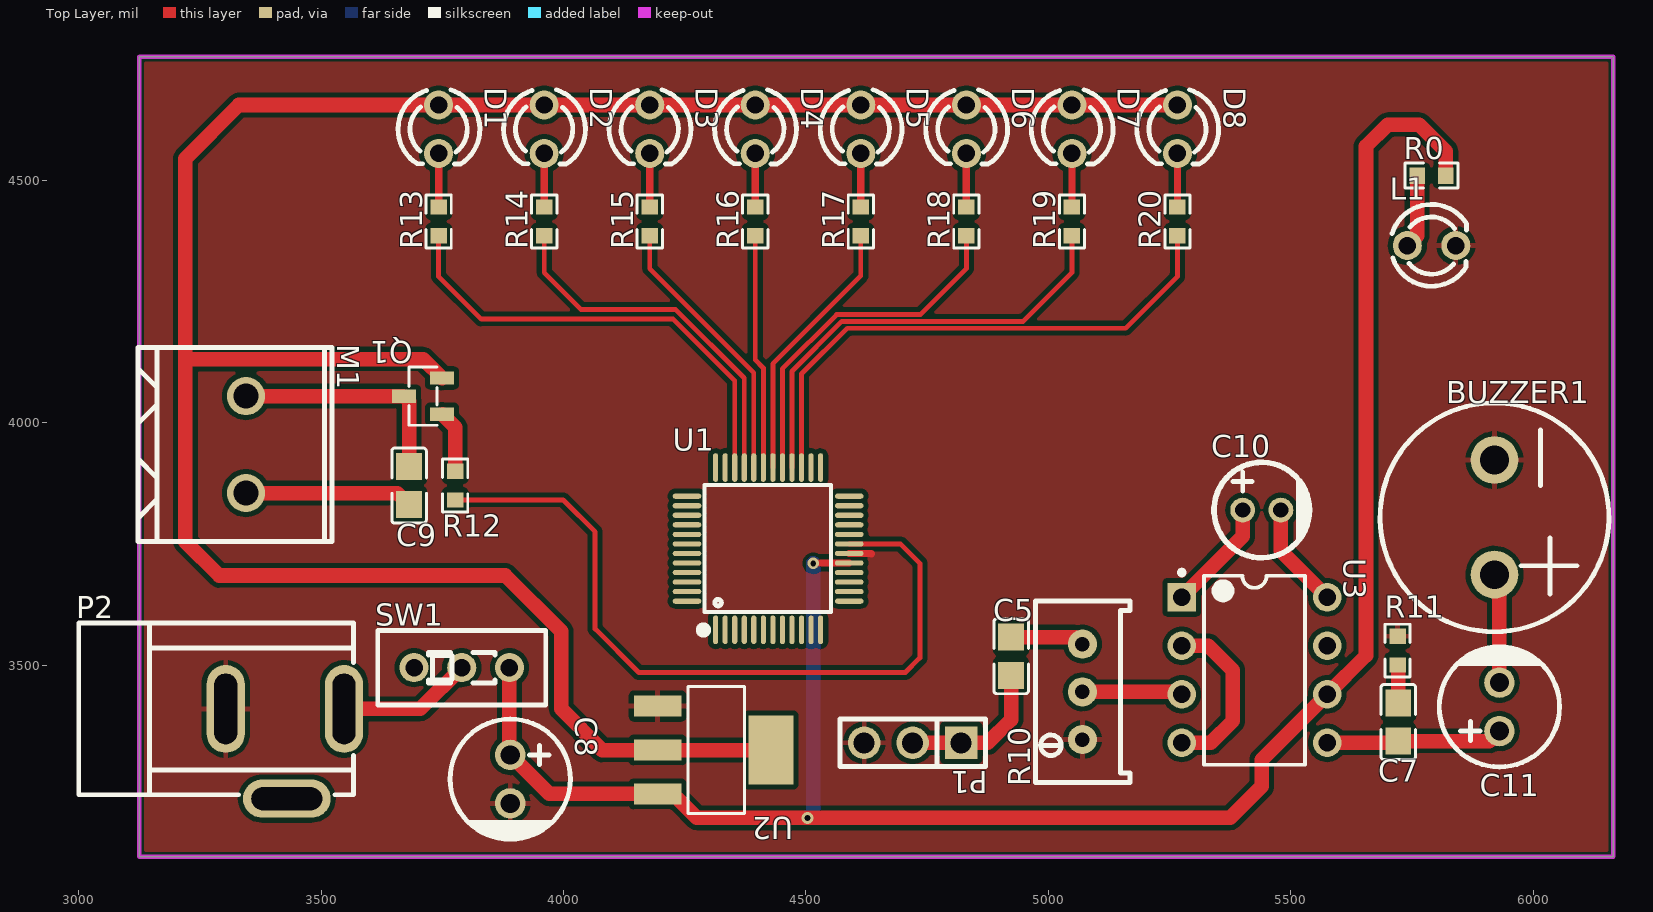
[diagram p0: Top Layer view]
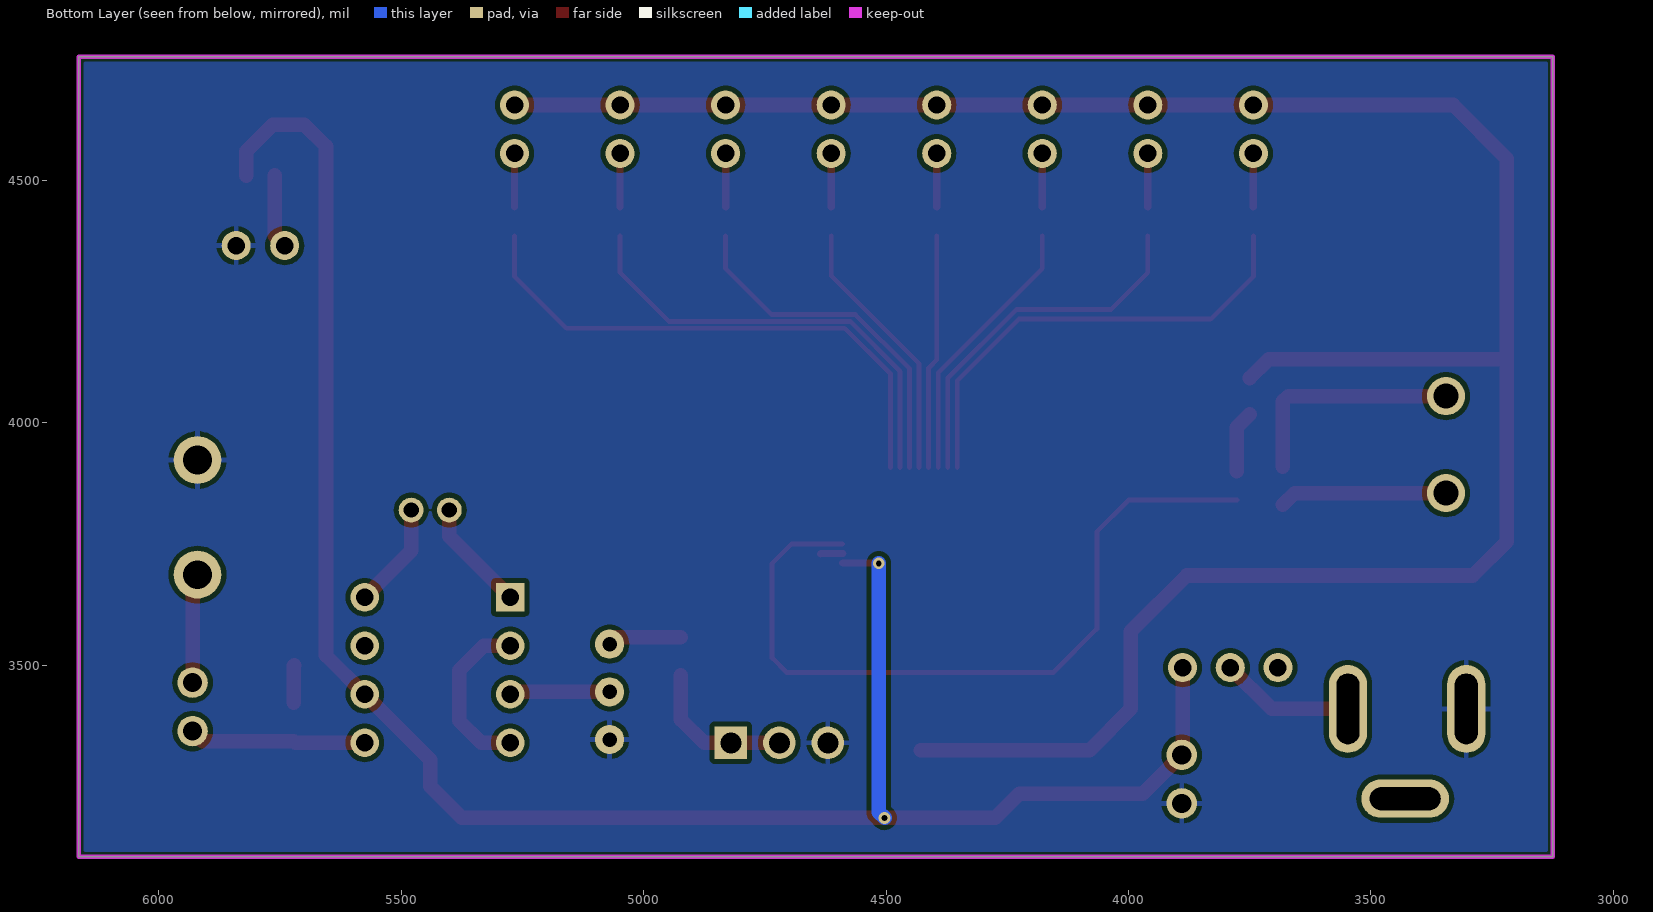
[diagram p1: Bottom Layer view, seen from below]
# Altium PCB MISC52120.pcbdoc
Units mil, origin at the board's own origin, x right, y up, seen from the top; angles counter-clockwise.
Board outline 3040 x 1650 mil, 2 copper layers (Top Layer, Bottom Layer), stack 62.206 mil thick; 36 components, 35 nets, 131 pads, 2 vias.

## Layer stack, top to bottom
Top Solder Mask Layer: solder mask 0.394, Dk 3.3
Top Layer: signal copper 1.379
Dielectric1: surface 59.449, FR4, Dk 4.5
Bottom Layer: signal copper 1.378
Bottom Solder Mask Layer: solder mask 0.394, Dk 3.3

## Board outline
3125,4755 3125,3105 6165,3105 6165,4755

## Design rules (kind name [scope] priority, off if disabled: settings)
BoardOutlineClearance copperThickness2oz_1 [All] p2 off: genericclearance=7.99 ignorepadtopadclearanceinfootprint=FALSE except(0: Arc-SplitContinuation Track-SplitContinuation SMDPad-SplitContinuation THPad-SplitContinuation Via-SplitContinuation Fill-SplitContinuation Region-SplitContinuation Poly-SplitContinuation Text-SplitContinuation Hole-SplitContinuation; 5.98: Arc-CutoutEdge Track-CutoutEdge SMDPad-CutoutEdge THPad-CutoutEdge Via-CutoutEdge Text-CutoutEdge; 6.9: Hole-OutlineEdge Hole-CutoutEdge; 10: Poly-OutlineEdge Poly-CutoutEdge; 11.81: Arc-OutlineEdge Track-OutlineEdge SMDPad-OutlineEdge THPad-OutlineEdge Via-OutlineEdge Fill-OutlineEdge Region-OutlineEdge Text-OutlineEdge Fill-CutoutEdge Region-CutoutEdge)
BoardOutlineClearance Plane_innerPlane_1 [All] p4 off: genericclearance=4.02 ignorepadtopadclearanceinfootprint=FALSE except(0: Arc-SplitContinuation Track-SplitContinuation SMDPad-SplitContinuation THPad-SplitContinuation Via-SplitContinuation Fill-SplitContinuation Region-SplitContinuation Poly-SplitContinuation Text-SplitContinuation Hole-SplitContinuation; 5.98: Arc-CutoutEdge Track-CutoutEdge SMDPad-CutoutEdge THPad-CutoutEdge Via-CutoutEdge Text-CutoutEdge; 6.9: Hole-OutlineEdge Hole-CutoutEdge; 10: Poly-OutlineEdge Poly-CutoutEdge; 11.81: Arc-OutlineEdge Track-OutlineEdge SMDPad-OutlineEdge THPad-OutlineEdge Via-OutlineEdge Fill-OutlineEdge Region-OutlineEdge Text-OutlineEdge Fill-CutoutEdge Region-CutoutEdge)
BoardOutlineClearance Copper_copperRegion_1 [All] p6 off: genericclearance=4.02 ignorepadtopadclearanceinfootprint=FALSE except(0: Arc-SplitContinuation Track-SplitContinuation SMDPad-SplitContinuation THPad-SplitContinuation Via-SplitContinuation Fill-SplitContinuation Region-SplitContinuation Poly-SplitContinuation Text-SplitContinuation Hole-SplitContinuation; 5.98: Arc-CutoutEdge Track-CutoutEdge SMDPad-CutoutEdge THPad-CutoutEdge Via-CutoutEdge Text-CutoutEdge; 6.9: Hole-OutlineEdge Hole-CutoutEdge; 10: Poly-OutlineEdge Poly-CutoutEdge; 11.81: Arc-OutlineEdge Track-OutlineEdge SMDPad-OutlineEdge THPad-OutlineEdge Via-OutlineEdge Fill-OutlineEdge Region-OutlineEdge Text-OutlineEdge Fill-CutoutEdge Region-CutoutEdge)
BoardOutlineClearance copperThickness1oz_1 [All] p8: genericclearance=4.02 ignorepadtopadclearanceinfootprint=FALSE except(0: Arc-SplitContinuation Track-SplitContinuation SMDPad-SplitContinuation THPad-SplitContinuation Via-SplitContinuation Fill-SplitContinuation Region-SplitContinuation Poly-SplitContinuation Text-SplitContinuation Hole-SplitContinuation; 5.98: Arc-CutoutEdge Track-CutoutEdge SMDPad-CutoutEdge THPad-CutoutEdge Via-CutoutEdge Text-CutoutEdge; 6.9: Hole-OutlineEdge Hole-CutoutEdge; 10: Poly-OutlineEdge Poly-CutoutEdge; 11.81: Arc-OutlineEdge Track-OutlineEdge SMDPad-OutlineEdge THPad-OutlineEdge Via-OutlineEdge Fill-OutlineEdge Region-OutlineEdge Text-OutlineEdge Fill-CutoutEdge Region-CutoutEdge)
Clearance copperThickness2oz [All] p1 off: gap=7.99 ignorepadtopadclearanceinfootprint=FALSE except(5.98: SMDPad-Track SMDPad-SMDPad THPad-Track SMDPad-THPad THPad-THPad Track-Via SMDPad-Via THPad-Via Via-Via Fill-SMDPad Region-SMDPad Fill-THPad Region-THPad Fill-Via Region-Via Fill-Fill Fill-Region Region-Region Arc-Track Arc-SMDPad Arc-THPad Arc-Via Fill-Arc Region-Arc Arc-Arc Text-Track SMDPad-Text Text-THPad Text-Via Fill-Text Region-Text Arc-Text Text-Text; 6.9: Hole-Track Hole-SMDPad Hole-THPad Hole-Via Fill-Hole Region-Hole Hole-Arc Hole-Text; 10: Poly-Track Poly-SMDPad Poly-THPad Poly-Via Poly-Fill Poly-Region Poly-Poly Poly-Arc Poly-Text Poly-Hole; 11.81: Fill-Track Region-Track)
Clearance Plane_innerPlane [All] p3 off: gap=4.02 ignorepadtopadclearanceinfootprint=FALSE except(5.98: SMDPad-Track SMDPad-SMDPad THPad-Track SMDPad-THPad THPad-THPad Track-Via SMDPad-Via THPad-Via Via-Via Fill-SMDPad Region-SMDPad Fill-THPad Region-THPad Fill-Via Region-Via Fill-Fill Fill-Region Region-Region Arc-Track Arc-SMDPad Arc-THPad Arc-Via Fill-Arc Region-Arc Arc-Arc Text-Track SMDPad-Text Text-THPad Text-Via Fill-Text Region-Text Arc-Text Text-Text; 6.9: Hole-Track Hole-SMDPad Hole-THPad Hole-Via Fill-Hole Region-Hole Hole-Arc Hole-Text; 10: Poly-Track Poly-SMDPad Poly-THPad Poly-Via Poly-Fill Poly-Region Poly-Poly Poly-Arc Poly-Text Poly-Hole; 11.81: Fill-Track Region-Track)
Clearance Copper_copperRegion [All] p5 off: gap=4.02 ignorepadtopadclearanceinfootprint=FALSE except(5.98: SMDPad-Track SMDPad-SMDPad THPad-Track SMDPad-THPad THPad-THPad Track-Via SMDPad-Via THPad-Via Via-Via Fill-SMDPad Region-SMDPad Fill-THPad Region-THPad Fill-Via Region-Via Fill-Fill Fill-Region Region-Region Arc-Track Arc-SMDPad Arc-THPad Arc-Via Fill-Arc Region-Arc Arc-Arc Text-Track SMDPad-Text Text-THPad Text-Via Fill-Text Region-Text Arc-Text Text-Text; 6.9: Hole-Track Hole-SMDPad Hole-THPad Hole-Via Fill-Hole Region-Hole Hole-Arc Hole-Text; 10: Poly-Track Poly-SMDPad Poly-THPad Poly-Via Poly-Fill Poly-Region Poly-Poly Poly-Arc Poly-Text Poly-Hole; 11.81: Fill-Track Region-Track)
Clearance copperThickness1oz [All] p7: gap=4.02 ignorepadtopadclearanceinfootprint=FALSE except(5.98: SMDPad-Track SMDPad-SMDPad THPad-Track SMDPad-THPad THPad-THPad Track-Via SMDPad-Via THPad-Via Via-Via Fill-SMDPad Region-SMDPad Fill-THPad Region-THPad Fill-Via Region-Via Fill-Fill Fill-Region Region-Region Arc-Track Arc-SMDPad Arc-THPad Arc-Via Fill-Arc Region-Arc Arc-Arc Text-Track SMDPad-Text Text-THPad Text-Via Fill-Text Region-Text Arc-Text Text-Text; 6.9: Hole-Track Hole-SMDPad Hole-THPad Hole-Via Fill-Hole Region-Hole Hole-Arc Hole-Text; 10: Poly-Track Poly-SMDPad Poly-THPad Poly-Via Poly-Fill Poly-Region Poly-Poly Poly-Arc Poly-Text Poly-Hole; 11.81: Fill-Track Region-Track)
DiffPairsRouting differentialPair [All] p1: maxlimit=6 minlimit=6 mostfreqgap=6 toplayer_minwidth=5 toplayer_prefwidth=10 toplayer_maxwidth=100 toplayer_mingap=6 toplayer_prefgap=6 toplayer_maxgap=6 bottomlayer_minwidth=5 bottomlayer_prefwidth=10 bottomlayer_maxwidth=100 bottomlayer_mingap=6 bottomlayer_prefgap=6 bottomlayer_maxgap=6 maxuncoupledlength=10
HoleToHoleClearance otherClearance [All] p1: gap=11.81 allowstackedmicrovias=TRUE
Length netLength [All] p1: minlimit=0 maxlimit=0
PasteMaskExpansion pasteMaskExpansion [All] p1: expansion=0
PlaneConnect innerPlane [All] p1: planeconnectstyle=Relief reliefexpansion=20 reliefentries=4 reliefconductorwidth=10 reliefairgap=10
PolygonConnect copperRegion [All] p1: connectstyle=Relief reliefconductorwidth=10 reliefentries=4 polygonreliefangle="90 Angle" airgapwidth=10 via.connectstyle=Relief via.reliefconductorwidth=10 via.reliefentries=4 via.polygonreliefangle="90 Angle" via.airgapwidth=10
RoutingVias viaSize [All] p1: holewidth=12.01 width=24.02 viastyle="Through Hole" minholewidth=11.81 minwidth=19.68 maxholewidth=248.03 maxwidth=393.7
SolderMaskExpansion solderMaskExpansion [IsVia] p1: expansion=-1000 istentingtop=TRUE
SolderMaskExpansion solderMaskExpansion [All] p2: expansion=2 istentingtop=FALSE
Width copperThickness2oz_2 [All] p1 off: maxlimit=100 minlimit=8 preferedwidth=10
Width copperThickness1oz_2 [All] p2: maxlimit=100 minlimit=5 preferedwidth=10

## Components (designator, comment, footprint, x,y, rotation, side; value= is the part's Value field where it differs from the comment)
BUZZER1 "buzzer" BUZ-TH_BD12.0-P6.00-D0.9-RD 5920,3805 r270 top
C5 "104" C0805 4923.07,3518.52 r270 top
C7 "104" C0805 5721.62,3382.82 r90 top
C8 "220uF" CAP-TH_BD6.3-P2.50-D1.0-FD 3890,3265 r270 top
C9 "104" C0805 3681.31,3870.47 r90 top
C10 "10uF" CAP-TH_BD5.0-P2.00-D0.8-FD 5440,3820 r0 top
C11 "220uF" CAP-TH_BD6.3-P2.50-D1.0-FD 5930.17,3414.15 r90 top
D1 "LED0" LED_TH-3mm 3742.34,4605.45 r270 top
D2 "LED0" LED_TH-3mm 3960.03,4605.45 r270 top
D3 "LED0" LED_TH-3mm 4177.71,4605.45 r270 top
D4 "LED0" LED_TH-3mm 4395.39,4605.45 r270 top
D5 "LED0" LED_TH-3mm 4613.07,4605.45 r270 top
D6 "LED0" LED_TH-3mm 4830.75,4605.45 r270 top
D7 "LED0" LED_TH-3mm 5048.44,4605.45 r270 top
D8 "LED0" LED_TH-3mm 5266.12,4605.45 r270 top
L1 "RED" LED_TH-3mm 5790.19,4365.45 r0 top
M1 "Motor" CONN-TH_2P-P5.08-WJ500V-5.08-2P 3345,3955 r270 top
P1 "" HDR-TH_3P-P2.54-V-M 4720,3340 r180 top
P2 "DC005" DC-IN-TH_DC005 3425.19,3317.31 r0 top
Q1 "9012" SOT-23-3_L2.9-W1.3-P1.90-LS2.4-BR 3710,4055 r0 top
R0 "1K" R0603 5790,4510 r0 top
R10 "10kΩ" R_3296 5065,3445 r90 top
R11 "4.7" R0603 5720,3530 r270 top
R12 "1K" R0603 3776.31,3870.47 r270 top
R13 "1K" R0603 3742.34,4415.34 r90 top
R14 "1K" R0603 3960.03,4415.34 r90 top
R15 "1K" R0603 4177.71,4415.34 r90 top
R16 "1K" R0603 4395.39,4415.34 r90 top
R17 "1K" R0603 4613.07,4415.34 r90 top
R18 "1K" R0603 4830.75,4415.34 r90 top
R19 "1K" R0603 5048.44,4415.34 r90 top
R20 "1K" R0603 5266.12,4415.34 r90 top
SW1 "Switch" SW-TH_SS-12D01-GX 3790,3495 r0 top
U1 "STM32F103" LQFP-48_L7.0-W7.0-P0.50-LS9.0-BL 4421.86,3740.34 r0 top
U2 "AMS1117" SOT-223-3_L6.5-W3.4-P2.30-LS7.0-BR 4310.89,3325 r180 top
U3 "LM386N-3/NOPB" DIP-8_L9.8-W6.6-P2.54-LS7.6-BL 5425,3490 r270 top

## Footprints (in the part's own frame and the unit in brackets; to place one, negate y for a bottom-side part, rotate by r counter-clockwise, add the part's x,y. Pads: shape width x height; smd on the part's side, far side on the other; paste and mask are expansions set on the pad)
BUZ-TH_BD12.0-P6.00-D0.9-RD [mm]
  round 2.5 hole 1.5 paste+0 mask+0.05: 1(-3,0) 2(3,0)
  silkscreen extent -5.99,-5.99 5.99,5.99
C0805 [mm]
  rect 1.41x1.35 smd paste-100 mask+0.051: 1(-1,0) 2(1,0)
  silkscreen extent -1.96,-0.9 1.96,0.9
CAP-TH_BD5.0-P2.00-D0.8-FD [mm]
  round 1.3 hole 0.8: 1(-1,0) 2(1,0)
  silkscreen extent -2.5,-2.5 2.5,2.5
CAP-TH_BD6.3-P2.50-D1.0-FD [mm]
  round 1.6 hole 1: 1(-1.27,0) 2(1.27,0)
  silkscreen extent -3.15,-3.15 3.17,3.15
CONN-TH_2P-P5.08-WJ500V-5.08-2P [mm]
  round 2 hole 1.3 copper offset 0,0 paste+0 mask+0.051: 1(-2.54,0) 2(2.54,0)
  silkscreen extent -5.08,-5.66 5.08,4.5
DC-IN-TH_DC005 [mm]
  oval 2x4.6 hole 1.2 slot 3.7 at 90 deg: 1(3.1,2.35) 2(-3.1,2.35)
  oval 4.6x2 hole 1.2 slot 3.7 at 0 deg: 3(0.1,-2.35)
  silkscreen extent -10.8,-2.15 3.6,6.85
DIP-8_L9.8-W6.6-P2.54-LS7.6-BL [mm]
  rect 1.5x1.5 hole 0.9: 1(-3.81,-3.81)
  round 1.5 hole 0.9: 2(-1.27,-3.81) 3(1.27,-3.81) 4(3.81,-3.81) 5(3.81,3.81) 6(1.27,3.81) 7(-1.27,3.81) 8(-3.81,3.81)
  silkscreen extent -5.23,-3.93 4.96,2.65
HDR-TH_3P-P2.54-V-M [mm]
  rect 1.7x1.7 hole 1.1: 1(-2.54,0)
  round 1.7 hole 1.1: 2(0,0) 3(2.54,0)
  silkscreen extent -3.81,-1.25 3.81,1.25
LED_TH-3mm [mil]
  round 60 hole 36 paste+0 mask+2: 1(-50,0) 2(50,0)
  silkscreen extent -81,-84 72,85
LQFP-48_L7.0-W7.0-P0.50-LS9.0-BL [mm]
  oval 0.27x1.5 smd paste+0 mask+0.05: 1(-2.75,-4.25) 2(-2.25,-4.25) 3(-1.75,-4.25) 4(-1.25,-4.25) 5(-0.75,-4.25) 6(-0.25,-4.25) 7(0.25,-4.25) 8(0.75,-4.25) 9(1.25,-4.25) 10(1.75,-4.25) 11(2.25,-4.25) 12(2.75,-4.25) 25(2.75,4.25) 26(2.25,4.25) 27(1.75,4.25) 28(1.25,4.25) 29(0.75,4.25) 30(0.25,4.25) 31(-0.25,4.25) 32(-0.75,4.25) 33(-1.25,4.25) 34(-1.75,4.25) 35(-2.25,4.25) 36(-2.75,4.25)
  oval 1.5x0.27 smd paste+0 mask+0.05: 13(4.25,-2.75) 14(4.25,-2.25) 15(4.25,-1.75) 16(4.25,-1.25) 17(4.25,-0.75) 18(4.25,-0.25) 19(4.25,0.25) 20(4.25,0.75) 21(4.25,1.25) 22(4.25,1.75) 23(4.25,2.25) 24(4.25,2.75) 37(-4.25,2.75) 38(-4.25,2.25) 39(-4.25,1.75) 40(-4.25,1.25) 41(-4.25,0.75) 42(-4.25,0.25) 43(-4.25,-0.25) 44(-4.25,-0.75) 45(-4.25,-1.25) 46(-4.25,-1.75) 47(-4.25,-2.25) 48(-4.25,-2.75)
  silkscreen extent -3.59,-4.46 3.3,3.34
R0603 [mil]
  rect 31.75x34.02 smd paste-3937.01 mask+2: 1(-29.66,0) 2(29.66,0)
  silkscreen extent -55,-26 55,26
R_3296 [mil]
  round 60 hole 30 paste+0 mask+2: 1(-98.4,-5) 2(0,-5) 3(98.4,-5)
  silkscreen extent -187,-103 187,92
SOT-23-3_L2.9-W1.3-P1.90-LS2.4-BR [mm]
  rect 1.25x0.7 smd: 1(1,-0.95) 2(1,0.95) 3(-1,0)
  silkscreen extent -0.73,-1.53 0.73,1.53
SOT-223-3_L6.5-W3.4-P2.30-LS7.0-BR [mm]
  rect 2.5x1.1 smd: 1(2.97,-2.3) 2(2.97,0) 3(2.97,2.3)
  rect 2.34x3.6 smd: 4(-2.97,0)
  silkscreen extent -1.57,-3.33 1.37,3.33
SW-TH_SS-12D01-GX [mil]
  round 60 hole 36: 1(-98.43,0) 2(-0.01,0) 3(98.42,0)
  silkscreen extent -173,-77 173,77

## Via types
v1: diameter 24, hole 12, Top Layer to Bottom Layer, 2 vias

## Nets (pads, with @x,y where several pads share a name; then routed paths per layer and width w, separated by ;. In a path a pad name is that pad's centre, name@x,y a point inside that pad or via, vN(x,y) a via of type N, cw(c..) or ccw(c..) an arc to the next point about the centre after c; other vN are vias at no path point)
3V: D1.1 D2.1 D3.1 D4.1 D5.1 D6.1 D7.1 D8.1 Q1.2 U2.2 U2.4 | length 4907
  Top Layer w30: Q1.2 3710.56,4131.21 3220,4131.21 ; U2.4 U2.2 4080,3325 3995,3410 3995,3570 3880,3685 3290,3685 3220,3755 3220,4131.21 ; D8.1 D7.1 D6.1 D5.1 D4.1 D3.1 D2.1 D1.1 3330.45,4655.45 3220,4545 3220,4131.21
$1N159: L1.1 R0.1 | length 152.9
  Top Layer w30: L1.1 5760.34,4385.6 R0.1
$1N348: Q1.1 R12.1 | length 128.6
  Top Layer w30: Q1.1 3776.31,3990.66 R12.1
$1N425: C9.2 M1.1 Q1.3 | length 475.2
  Top Layer w30: M1.1 Q1.3 ; Q1.3 3681.31,4044.32 C9.2
$1N506: C9.1 M1.2 | length 346.2
  Top Layer w30: M1.2 3657.42,3854.99 C9.1
$1N2273: D1.2 R13.2 | length 110.4
  Top Layer w15: R13.2 D1.2
$1N2330: D2.2 R14.2 | length 110.4
  Top Layer w15: R14.2 D2.2
$1N2379: D3.2 R15.2 | length 110.4
  Top Layer w15: R15.2 D3.2
$1N2428: D4.2 R16.2 | length 110.4
  Top Layer w15: R16.2 D4.2
$1N2477: D5.2 R17.2 | length 110.4
  Top Layer w15: R17.2 D5.2
$1N2526: D6.2 R18.2 | length 110.4
  Top Layer w15: R18.2 D6.2
$1N2575: D7.2 R19.2 | length 110.4
  Top Layer w15: R19.2 D7.2
$1N2624: D8.2 R20.2 | length 110.4
  Top Layer w15: R20.2 D8.2
$1N4137: P2.1 SW1.2 | length 278
  Top Layer w30: P2.1 3704.82,3409.83 SW1.2
$1N5014: C5.2 P1.1 P1.2 | length 314.1
  Top Layer w30: P1.2 P1.1 4875,3340 4923.07,3388.07 C5.2
$1N5054: C5.1 R10.3 | length 152.9
  Top Layer w30: C5.1 5055.51,3557.89 R10.3
$1N5291: R10.2 U3.3 | length 207.1
  Top Layer w30: R10.2 5270,3445 U3.3
$1N5301: U3.2 U3.4 | length 354.4
  Top Layer w30: U3.4 5335,3340 5380,3385 5380,3490 5330,3540 U3.2
$1N5514: C10.1 U3.1 | length 232
  Top Layer w30: U3.1 5400.63,3765.63 C10.1
$1N5523: C10.2 U3.8 | length 219.6
  Top Layer w30: C10.2 5479.37,3735.63 U3.8
$1N5581: C7.1 C11.1 U3.5 | length 365.2
  Top Layer w30: U3.5 5718.17,3340 C7.1 5909.48,3343.45 C11.1
$1N5607: C7.2 R11.2 | length 78.8
  Top Layer w30: R11.2 5721.62,3498.72 C7.2
$1N5737: BUZZER1.2 C11.2 | length 227
  Top Layer w30: BUZZER1.2 5930.17,3676.72 C11.2
GND: BUZZER1.1 C8.2 L1.2 P1.3 P2.2 R10.1 R11.1 U1.18 U2.1 | length 46
  Top Layer w15: U1.18 4634.5,3730.5 4635,3730
PA0: U1.23
PA4: R20.1 U1.27 | length 1135.7
  Top Layer w10: U1.27 4490.76,4100.76 4585,4195 5159.52,4195 5266.12,4301.59 R20.1
PA5: R19.1 U1.28 | length 936.1
  Top Layer w10: U1.28 4471.07,4106.07 4574.02,4209.02 4947.7,4209.02 5048.44,4309.75 R19.1
PA6: R18.1 U1.29 | length 736.4
  Top Layer w10: U1.29 4451.39,4111.39 4563.03,4223.03 4735.88,4223.03 4830.75,4317.9 R18.1
PA7: R17.1 U1.30 | length 553.1
  Top Layer w10: U1.30 4431.7,4121.7 4613.07,4303.07 R17.1
PB0: R16.1 U1.31 | length 484.9
  Top Layer w10: R16.1 4395.39,4129.61 4412.02,4112.98 U1.31
PB1: R15.1 U1.32 | length 566.9
  Top Layer w10: R15.1 4177.71,4317.9 4392.33,4103.28 U1.32
PB8: R12.2 U1.19 | length 1593.1
  Top Layer w10: R12.2 3999.19,3840.81 4065,3775 4065,3575 4155,3485 4705,3485 4735,3515 4735,3710 4694.82,3750.18 U1.19
PB10: R14.1 U1.33 | length 763.3
  Top Layer w10: R14.1 3960.03,4309.75 4036.28,4233.49 4231.51,4233.49 4372.65,4092.35 U1.33
PB11: R13.1 U1.34 | length 963
  Top Layer w10: R13.1 3742.34,4301.59 3830.14,4213.8 4226.2,4213.8 4352.96,4087.04 U1.34
VCC: C8.1 R0.2 SW1.3 U1.17 U2.3 U3.6 | length 4081.2
  Top Layer w15: v1(4515,3710) 4515.81,3710.81 U1.17
  Top Layer w30: SW1.3 3888.43,3316.57 C8.1 3970.55,3234.45 U2.3 4225.55,3234.45 4275,3185 v1(4503,3185) 5375,3185 5440,3250 5440,3305 U3.6 5655,3520 5655,4570 5700,4615 5765,4615 5819.66,4560.34 R0.2
  Bottom Layer w30: v1(4503,3185) 4515,3197 v1(4515,3710)
pads on no net: P2.3 SW1.1 U1.1 U1.2 U1.3 U1.4 U1.5 U1.6 U1.7 U1.8 U1.9 U1.10 U1.11 U1.12 U1.13 U1.14 U1.15 U1.16 U1.20 U1.21 U1.22 U1.24 U1.25 U1.26 U1.35 U1.36 U1.37 U1.38 U1.39 U1.40 U1.41 U1.42 U1.43 U1.44 U1.45 U1.46 U1.47 U1.48 U3.7

## Polygon pours and split planes (outlines as drawn)
GND on Top Layer (solid, remove dead copper, pour order 0): 3055,4870 3055,3010 6250,3010 6250,4870
GND on Bottom Layer (solid, remove dead copper, pour order 2): 3080,4805 3080,3000 6270,3000 6270,4805

## Keep-outs
Board Outline Layer:
  the board outline again, w10